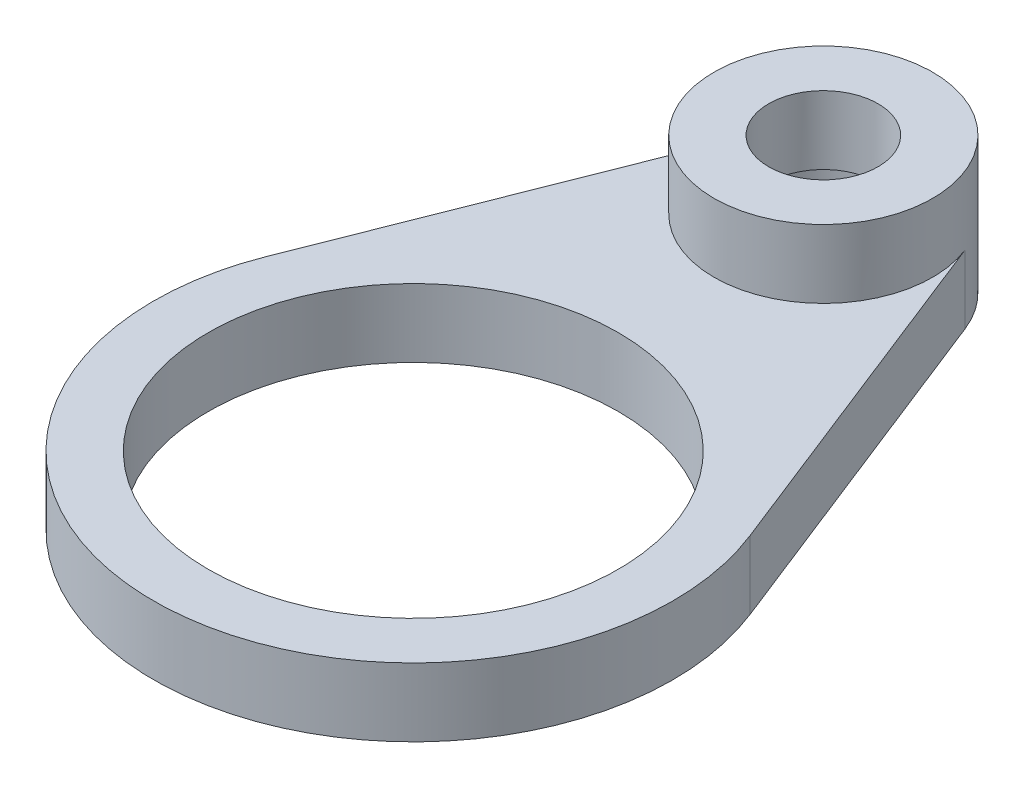
from build123d import *

# Parameters (mm, degrees)
BOSS_EXTRUDE1_DEPTH = 5
SKETCH2_R           = 8
BOSS_EXTRUDE2_DEPTH = 5
SKETCH3_R           = 4
SKETCH3_R_2         = 15
CUT_EXTRUDE1_DEPTH  = 39
SKETCH4_R           = 4.5
CUT_EXTRUDE2_DEPTH  = 5


with BuildPart() as part:
    # Sketch1 → Boss-Extrude1 (new body)
    with BuildSketch(Plane(origin=(0, 0, 0), x_dir=(1, 0, 0), z_dir=(0, 1, 0))):
        with BuildLine():
            Line((-7.44281906, 2.933333333), (-17.676695267, -23.033333333))
            ThreePointArc((-17.676695267, -23.033333333), (0, -49), (17.676695267, -23.033333333))
            Line((17.676695267, -23.033333333), (7.44281906, 2.933333333))
            ThreePointArc((7.44281906, 2.933333333), (0, 8), (-7.44281906, 2.933333333))
        make_face()
    extrude(amount=BOSS_EXTRUDE1_DEPTH)

    # Sketch2 → Boss-Extrude2 (add)
    with BuildSketch(Plane(origin=(0, 5, 0), x_dir=(1, 0, 0), z_dir=(0, 1, 0))):
        with Locations(Location((0, 0, 0), (0, 0, 158.489811733))):
            Circle(SKETCH2_R)
    extrude(amount=BOSS_EXTRUDE2_DEPTH)

    # Sketch3 → Cut-Extrude1 (cut)
    with BuildSketch(Plane(origin=(0, 10, 0), x_dir=(1, 0, 0), z_dir=(0, 1, 0))):
        with Locations(Location((0, 0, 0), (0, 0, 270))):
            Circle(SKETCH3_R)
        with Locations(Location((0, -30, 0), (0, 0, 270))):
            Circle(SKETCH3_R_2)
    extrude(amount=-CUT_EXTRUDE1_DEPTH, mode=Mode.SUBTRACT)

    # Sketch4 → Cut-Extrude2 (cut)
    with BuildSketch(Plane.XZ):
        with Locations(Location((0, 0, 0), (0, 0, 270))):
            Circle(SKETCH4_R)
    extrude(amount=-CUT_EXTRUDE2_DEPTH, mode=Mode.SUBTRACT)


solid = part.part
